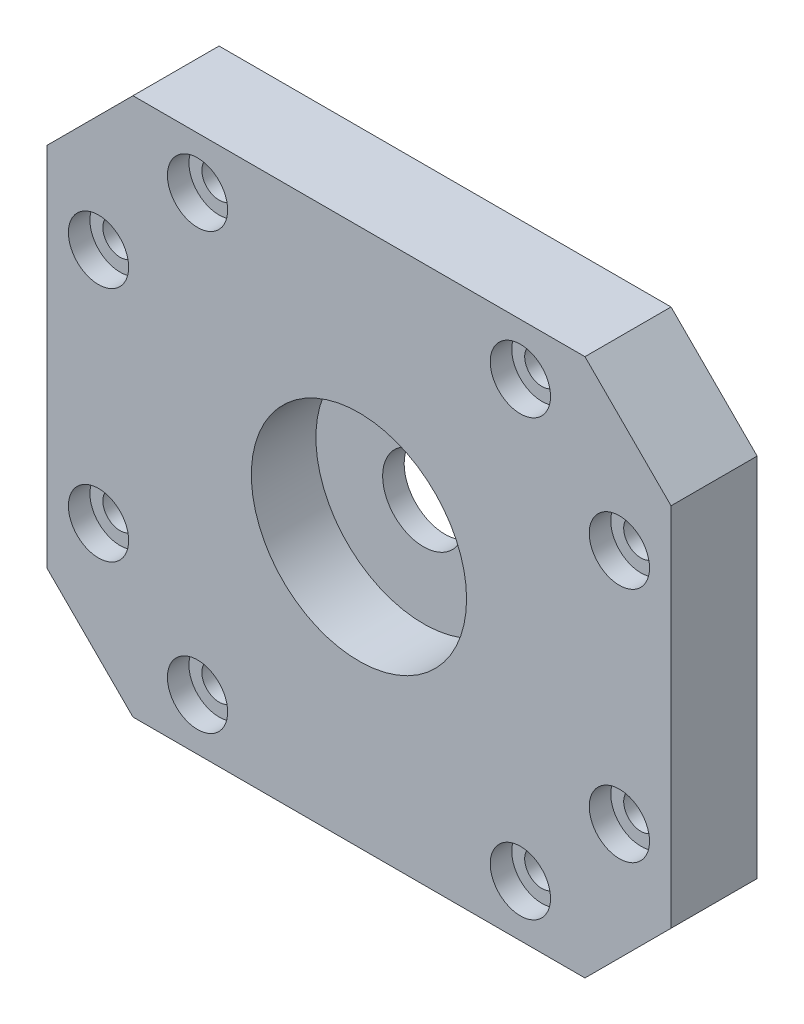
from build123d import *

# Parameters (mm, degrees)
SKETCH_1_W          = 145
SKETCH_1_H          = 125
EXTRUDE_1_DEPTH     = 20
CHAMFER_1_SIZE      = 20
SKETCH_2_R          = 7
CUT_EXTRUDE_1_DEPTH = 5
CUT_EXTRUDE_2_REACH = 98.889
SKETCH_3_R          = 4
CUT_EXTRUDE_5_REACH = 99.788
SKETCH_6_R          = 9.5
SKETCH_7_R          = 25
CUT_EXTRUDE_6_DEPTH = 15


with BuildPart() as part:
    # 草图1 → 凸台-拉伸1 (new body)
    with BuildSketch(Plane.XY):
        Rectangle(SKETCH_1_W, SKETCH_1_H)
    extrude(amount=EXTRUDE_1_DEPTH)

    # 倒角1
    chamfer_1_edges = [part.edges().sort_by_distance(p)[0] for p in [
        (72.5, -62.5, 10),
        (-72.5, -62.5, 10),
        (-72.5, 62.5, 10),
        (72.5, 62.5, 10),
    ]]
    chamfer(chamfer_1_edges, length=CHAMFER_1_SIZE)

    # 草图2 → 切除-拉伸1 (cut)
    with BuildSketch(Plane.XY.offset(20)):
        with Locations((-37.5, 50.5)):
            Circle(SKETCH_2_R)
        with Locations((37.5, 50.5)):
            Circle(SKETCH_2_R)
        with Locations((-60.5, 27.5)):
            Circle(SKETCH_2_R)
        with Locations((-60.5, -27.5)):
            Circle(SKETCH_2_R)
        with Locations((-37.5, -50.5)):
            Circle(SKETCH_2_R)
        with Locations((37.5, -50.5)):
            Circle(SKETCH_2_R)
        with Locations((60.5, 27.5)):
            Circle(SKETCH_2_R)
        with Locations((60.5, -27.5)):
            Circle(SKETCH_2_R)
    extrude(amount=-CUT_EXTRUDE_1_DEPTH, mode=Mode.SUBTRACT)

    # 草图3 → 切除-拉伸2 (cut, up to next)
    with BuildSketch(Plane.XY.offset(15), mode=Mode.PRIVATE) as cut_extrude_2_sk1:
        with Locations((-37.5, 50.5)):
            Circle(SKETCH_3_R)
    cut_extrude_2_tool1 = extrude(cut_extrude_2_sk1.sketch, amount=-CUT_EXTRUDE_2_REACH, mode=Mode.PRIVATE) & part.part
    # 草图3 → 切除-拉伸2 (cut, up to next)
    with BuildSketch(Plane.XY.offset(15), mode=Mode.PRIVATE) as cut_extrude_2_sk2:
        with Locations((-60.5, 27.5)):
            Circle(SKETCH_3_R)
    cut_extrude_2_tool2 = extrude(cut_extrude_2_sk2.sketch, amount=-CUT_EXTRUDE_2_REACH, mode=Mode.PRIVATE) & part.part
    # 草图3 → 切除-拉伸2 (cut, up to next)
    with BuildSketch(Plane.XY.offset(15), mode=Mode.PRIVATE) as cut_extrude_2_sk3:
        with Locations((-60.5, -27.5)):
            Circle(SKETCH_3_R)
    cut_extrude_2_tool3 = extrude(cut_extrude_2_sk3.sketch, amount=-CUT_EXTRUDE_2_REACH, mode=Mode.PRIVATE) & part.part
    # 草图3 → 切除-拉伸2 (cut, up to next)
    with BuildSketch(Plane.XY.offset(15), mode=Mode.PRIVATE) as cut_extrude_2_sk4:
        with Locations((-37.5, -50.5)):
            Circle(SKETCH_3_R)
    cut_extrude_2_tool4 = extrude(cut_extrude_2_sk4.sketch, amount=-CUT_EXTRUDE_2_REACH, mode=Mode.PRIVATE) & part.part
    # 草图3 → 切除-拉伸2 (cut, up to next)
    with BuildSketch(Plane.XY.offset(15), mode=Mode.PRIVATE) as cut_extrude_2_sk5:
        with Locations((37.5, 50.5)):
            Circle(SKETCH_3_R)
    cut_extrude_2_tool5 = extrude(cut_extrude_2_sk5.sketch, amount=-CUT_EXTRUDE_2_REACH, mode=Mode.PRIVATE) & part.part
    # 草图3 → 切除-拉伸2 (cut, up to next)
    with BuildSketch(Plane.XY.offset(15), mode=Mode.PRIVATE) as cut_extrude_2_sk6:
        with Locations((60.5, 27.5)):
            Circle(SKETCH_3_R)
    cut_extrude_2_tool6 = extrude(cut_extrude_2_sk6.sketch, amount=-CUT_EXTRUDE_2_REACH, mode=Mode.PRIVATE) & part.part
    # 草图3 → 切除-拉伸2 (cut, up to next)
    with BuildSketch(Plane.XY.offset(15), mode=Mode.PRIVATE) as cut_extrude_2_sk7:
        with Locations((60.5, -27.5)):
            Circle(SKETCH_3_R)
    cut_extrude_2_tool7 = extrude(cut_extrude_2_sk7.sketch, amount=-CUT_EXTRUDE_2_REACH, mode=Mode.PRIVATE) & part.part
    # 草图3 → 切除-拉伸2 (cut, up to next)
    with BuildSketch(Plane.XY.offset(15), mode=Mode.PRIVATE) as cut_extrude_2_sk8:
        with Locations((37.5, -50.5)):
            Circle(SKETCH_3_R)
    cut_extrude_2_tool8 = extrude(cut_extrude_2_sk8.sketch, amount=-CUT_EXTRUDE_2_REACH, mode=Mode.PRIVATE) & part.part
    add(cut_extrude_2_tool1.solids().sort_by_distance((-37.5, 50.5, 15))[0], mode=Mode.SUBTRACT)
    add(cut_extrude_2_tool2.solids().sort_by_distance((-60.5, 27.5, 15))[0], mode=Mode.SUBTRACT)
    add(cut_extrude_2_tool3.solids().sort_by_distance((-60.5, -27.5, 15))[0], mode=Mode.SUBTRACT)
    add(cut_extrude_2_tool4.solids().sort_by_distance((-37.5, -50.5, 15))[0], mode=Mode.SUBTRACT)
    add(cut_extrude_2_tool5.solids().sort_by_distance((37.5, 50.5, 15))[0], mode=Mode.SUBTRACT)
    add(cut_extrude_2_tool6.solids().sort_by_distance((60.5, 27.5, 15))[0], mode=Mode.SUBTRACT)
    add(cut_extrude_2_tool7.solids().sort_by_distance((60.5, -27.5, 15))[0], mode=Mode.SUBTRACT)
    add(cut_extrude_2_tool8.solids().sort_by_distance((37.5, -50.5, 15))[0], mode=Mode.SUBTRACT)

    # 草图6 → 切除-拉伸5 (cut, up to next)
    with BuildSketch(Plane(origin=(0, 0, 0), x_dir=(-1, 0, 0), z_dir=(0, 0, -1)), mode=Mode.PRIVATE) as cut_extrude_5_sk1:
        Circle(SKETCH_6_R)
    cut_extrude_5_tool1 = extrude(cut_extrude_5_sk1.sketch, amount=-CUT_EXTRUDE_5_REACH, mode=Mode.PRIVATE) & part.part
    add(cut_extrude_5_tool1.solids().sort_by_distance((0, 0, 0))[0], mode=Mode.SUBTRACT)

    # 草图7 → 切除-拉伸6 (cut)
    with BuildSketch(Plane.XY.offset(20)):
        Circle(SKETCH_7_R)
    extrude(amount=-CUT_EXTRUDE_6_DEPTH, mode=Mode.SUBTRACT)


solid = part.part
